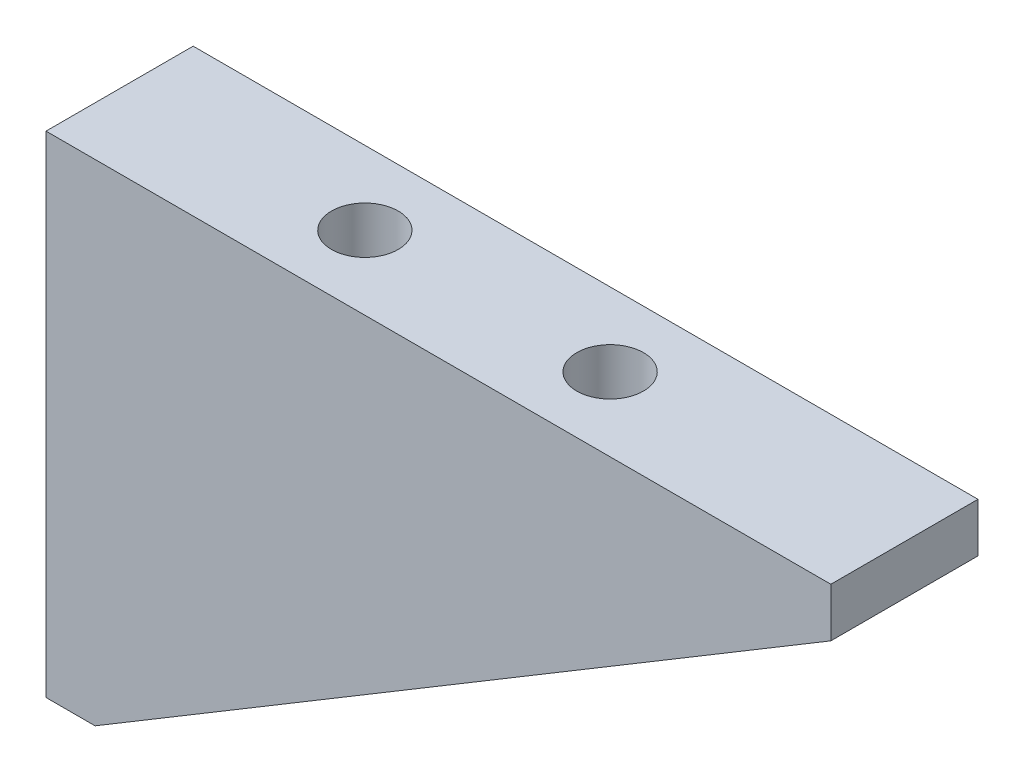
SolidWorks part; units mm, degrees
ref_plane "Front Plane" through (0, 0, 0) normal (0, 0, 1) x (1, 0, 0)
ref_plane "Top Plane" through (0, 0, 0) normal (0, 1, 0) x (1, 0, 0)
ref_plane "Right Plane" through (0, 0, 0) normal (1, 0, 0) x (0, 0, -1)
sketch "Sketch1" plane through (0, 0, 0) normal (0, 0, 1) x (1, 0, 0)
  line L0 (0, 0) -> (0, 50)
  line L1 (0, 50) -> (80, 50)
  line L2 (80, 50) -> (80, 45)
  line L3 (80, 45) -> (5, 0)
  line L4 (5, 0) -> (0, 0)
  dimension "D1" = 80
  dimension "D2" = 50
  dimension "D3" = 5
  dimension "D4" = 5
extrude "Boss-Extrude1" add sketch "Sketch1" along normal blind 15
hole_wizard "M8 Tapped Hole1" positions "Sketch3" profile "Sketch2" tap size "M8" standard "Iso"
sketch "Sketch3" plane through (0, 50, 0) normal (0, 1, 0) x (1, 0, 0)
  line L0 (0, -15) -> (0, 0) construction
  line L1 (0, -7.5) -> (52.1208, -7.5) construction
  point P0 (25, -7.5)
  point P2 (50, -7.5)
  dimension "D1" = 25
  dimension "D2" = 25
sketch "Sketch2" plane through (25, 50, 7.5) normal (1, 0, 0) x (0, 0, 1)
  line L0 (0, 0) -> (0, 24.2929)
  line L1 (0, 24.2929) -> (3.4, 22.25)
  line L2 (3.4, 22.25) -> (3.4, 0)
  line L5 (3.4, 0) -> (0, 0)
  line L10 (0, 24.2929) -> (-3.4, 22.25) construction
  line L11 (0, -6.35) -> (0, 107.95) construction
  dimension "螺纹孔钻头直径" = 6.8
  dimension "螺纹孔钻头深度" = 22.25
  dimension "导头角度" = 118
cosmetic thread "Cosmetic Thread1"
cosmetic thread "Cosmetic Thread2"
hole_wizard "M8 Tapped Hole2" positions "Sketch5" profile "Sketch4" tap size "M8" standard "Iso"
sketch "Sketch5" plane through (0, 0, 0) normal (-1, 0, 0) x (0, 0, 1)
  line L0 (0, 25) -> (19.4581, 25) construction
  line L1 (0, 50) -> (0, 0) construction
  line L3 (7.5, 50) -> (7.5, 2.721) construction
  line L4 (15, 50) -> (0, 50) construction
  point P0 (7.5, 35)
  point P2 (7.5, 15)
  dimension "D1" = 20
sketch "Sketch4" plane through (0, 35, 7.5) normal (0, 1, 0) x (0, 0, 1)
  line L0 (0, 0) -> (0, 24.2929)
  line L1 (0, 24.2929) -> (3.4, 22.25)
  line L2 (3.4, 22.25) -> (3.4, 0)
  line L5 (3.4, 0) -> (0, 0)
  line L10 (0, 24.2929) -> (-3.4, 22.25) construction
  line L11 (0, -6.35) -> (0, 107.95) construction
  dimension "螺纹孔钻头直径" = 6.8
  dimension "螺纹孔钻头深度" = 22.25
  dimension "导头角度" = 118
cosmetic thread "Cosmetic Thread3"
cosmetic thread "Cosmetic Thread4"
